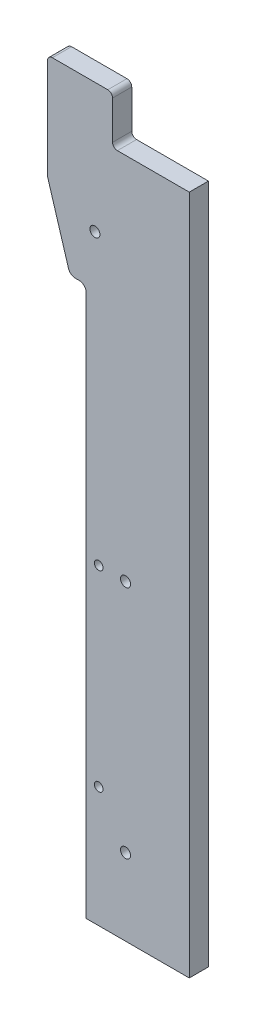
SolidWorks part; units mm, degrees
material "Q235B"
ref_plane "Front Plane" through (0, 0, 0) normal (0, 0, 1) x (1, 0, 0)
ref_plane "Top Plane" through (0, 0, 0) normal (0, 1, 0) x (1, 0, 0)
ref_plane "Right Plane" through (0, 0, 0) normal (1, 0, 0) x (0, 0, -1)
sketch "Sketch1" plane through (0, 0, 0) normal (0, 0, 1) x (1, 0, 0)
  line L0 (0, 0) -> (0, 1145.5161)
  line L1 (-80.68, 1300) -> (-80.68, 1520)
  line L2 (215, 1420) -> (215, 0)
  line L3 (215, 0) -> (0, 0)
  line L4 (-33.7239, 1145.5161) -> (-80.68, 1300)
  line L5 (-33.7239, 1145.5161) -> (0, 1145.5161)
  line L6 (215, 1420) -> (55, 1420)
  line L7 (55, 1420) -> (55, 1520)
  line L8 (55, 1520) -> (-80.68, 1520)
  circle A0 centre (26, 251) radius 9
  circle A1 centre (26, 651) radius 9
  dimension "D6" = 18
  dimension "D8" = 400
  dimension "D9" = 26
  dimension "D1" = 215
  dimension "D2" = 1145.5161
  dimension "D3" = 154.4839
  dimension "D4" = 1420
  dimension "D5" = 33.7239
  dimension "D7" = 251
  dimension "D10" = 295.68
  dimension "D11" = 100
  dimension "D12" = 160
extrude "Boss-Extrude1" add sketch "Sketch1" along normal blind 40
hole_wizard "M24 Tapped Hole1" positions "3DSketch1" profile "Sketch2" tap size "M24" standard "GB" end condition up to next
sketch3d "3DSketch1"
  line L0 (-80.68, 1300, 0) -> (-33.7217, 1145.5168, 0) construction
  line L1 (0, 0, 0) -> (215, 0, 0) construction
  line L3 (0, 1145.5161, 0) -> (0, 0, 0) construction
  point P0 (18.1328, 1250, 0)
  point P7 (82, 650, 0)
  point P9 (82, 160, 0)
  dimension "D1" = 80
  dimension "D2" = 1250
  dimension "D3" = 82
  dimension "D4" = 82
  dimension "D5" = 160
  dimension "D6" = 650
sketch "Sketch2" plane through (18.1328, 1250, 0) normal (1, 0, 0) x (0, 1, 0)
  line L0 (0, 0) -> (0, 40)
  line L1 (0, 40) -> (10.5, 40)
  line L2 (10.5, 40) -> (10.5, 0)
  line L5 (10.5, 0) -> (0, 0)
  line L11 (0, -6.35) -> (0, 107.95) construction
  dimension "通孔螺纹孔钻头直径" = 21
  dimension "通孔螺纹孔钻头深度" = 40
cosmetic thread "Hole thread 1" parameters "D2"=24
cosmetic thread "Hole thread 2" parameters "D2"=24
cosmetic thread "Hole thread 3" parameters "D2"=24
fillet "Fillet1" radius 15 2 edges at (0, 1145.5161, 20) (-33.7239, 1145.5161, 20)
fillet "Fillet2" radius 10 3 edges at (-80.68, 1520, 20) (55, 1520, 20) (55, 1420, 20)
